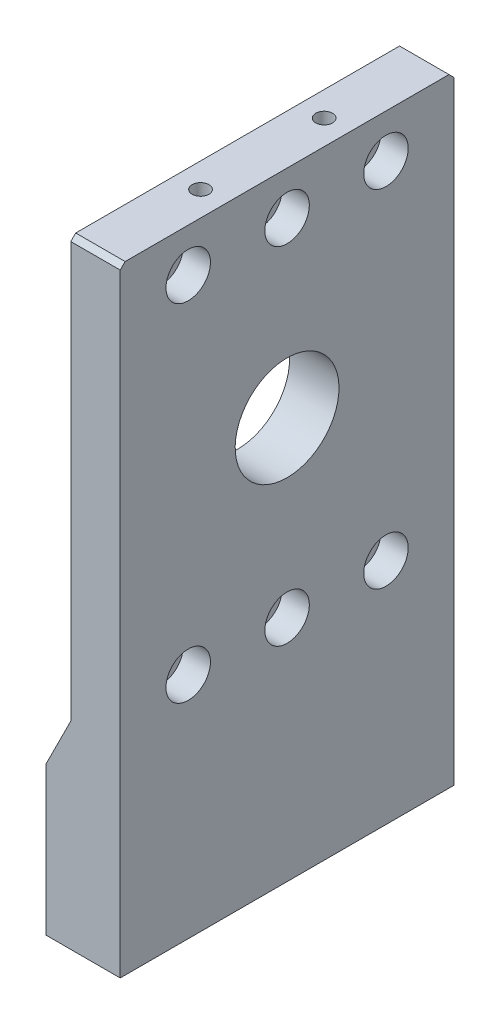
from build123d import *

# Parameters (mm, degrees)
BOSS_EXTRUDE1_DEPTH                                  = 67.5
M8_TAPPED_HOLE1_D                                    = 6.8
M8_TAPPED_HOLE1_DEPTH                                = 19.75
M8_TAPPED_HOLE1_TIP                                  = 2.042926105
HOLE_SIZE_PER_SOCKET_HEAD_CAP_SCREW_TYPE_D           = 11
HOLE_SIZE_PER_SOCKET_HEAD_CAP_SCREW_TYPE_CBORE_D     = 18
HOLE_SIZE_PER_SOCKET_HEAD_CAP_SCREW_TYPE_CBORE_DEPTH = 11
SKETCH8_R                                            = 21
CUT_EXTRUDE1_DEPTH                                   = 260.723410574
M8_TAPPED_HOLE2_D                                    = 6.8
M8_TAPPED_HOLE2_DEPTH                                = 19.75
M8_TAPPED_HOLE2_TIP                                  = 2.042926105
CHAMFER1_SIZE                                        = 2
M3_TAPPED_HOLE1_D                                    = 2.5
M3_TAPPED_HOLE1_DEPTH                                = 7.5
M3_TAPPED_HOLE1_TIP                                  = 0.751075774


with BuildPart() as part:
    # Sketch1 → Boss-Extrude1 (new, symmetric)
    with BuildSketch(Plane.XY):
        Polygon((0, 0), (0, 60), (10, 80), (10, 250), (30, 250), (30, 0), align=None)
    extrude(amount=BOSS_EXTRUDE1_DEPTH, both=True)

    # M8 Tapped Hole1
    with Locations(Plane.XZ):
        with Locations((6, -42.5), (24, -42.5), (24, 0), (6, 0), (6, 42.5), (24, 42.5)):
            Hole(M8_TAPPED_HOLE1_D / 2, depth=M8_TAPPED_HOLE1_DEPTH)
            with Locations((0, 0, -(M8_TAPPED_HOLE1_DEPTH + M8_TAPPED_HOLE1_TIP / 2))):  # 118° drill point
                Cone(0, M8_TAPPED_HOLE1_D / 2, M8_TAPPED_HOLE1_TIP, mode=Mode.SUBTRACT)

    # Hole size per socket head cap screw type1 (through all)
    with Locations(Plane(origin=(30, 0, 0), x_dir=(0, 0, -1), z_dir=(1, 0, 0))):
        with Locations((-40, 232.5), (40, 232.5), (40, 92.5), (-40, 92.5), (0, 232.5), (0, 92.5)):
            CounterBoreHole(HOLE_SIZE_PER_SOCKET_HEAD_CAP_SCREW_TYPE_D / 2, HOLE_SIZE_PER_SOCKET_HEAD_CAP_SCREW_TYPE_CBORE_D / 2, HOLE_SIZE_PER_SOCKET_HEAD_CAP_SCREW_TYPE_CBORE_DEPTH)

    # Sketch8 → Cut-Extrude1 (cut, through all)
    with BuildSketch(Plane.ZY.offset(-10)):
        with Locations(Location((0, 162.5, 0), (0, 0, 270))):
            Circle(SKETCH8_R)
    extrude(amount=-CUT_EXTRUDE1_DEPTH, mode=Mode.SUBTRACT)

    # M8 Tapped Hole2
    with Locations(Plane(origin=(0, 250, 0), x_dir=(-1, 0, 0), z_dir=(0, 1, 0))):
        with Locations((-20, -25), (-20, 25)):
            Hole(M8_TAPPED_HOLE2_D / 2, depth=M8_TAPPED_HOLE2_DEPTH)
            with Locations((0, 0, -(M8_TAPPED_HOLE2_DEPTH + M8_TAPPED_HOLE2_TIP / 2))):  # 118° drill point
                Cone(0, M8_TAPPED_HOLE2_D / 2, M8_TAPPED_HOLE2_TIP, mode=Mode.SUBTRACT)

    # Chamfer1
    chamfer1_edges = [part.edges().sort_by_distance(p)[0] for p in [
        (20, 250, 67.5),
        (20, 250, -67.5),
    ]]
    chamfer(chamfer1_edges, length=CHAMFER1_SIZE)

    # M3 Tapped Hole1
    with Locations(Plane.ZY.offset(-10)):
        with Locations((-37.5, 152.5), (-37.5, 172.5)):
            Hole(M3_TAPPED_HOLE1_D / 2, depth=M3_TAPPED_HOLE1_DEPTH)
            with Locations((0, 0, -(M3_TAPPED_HOLE1_DEPTH + M3_TAPPED_HOLE1_TIP / 2))):  # 118° drill point
                Cone(0, M3_TAPPED_HOLE1_D / 2, M3_TAPPED_HOLE1_TIP, mode=Mode.SUBTRACT)


solid = part.part
